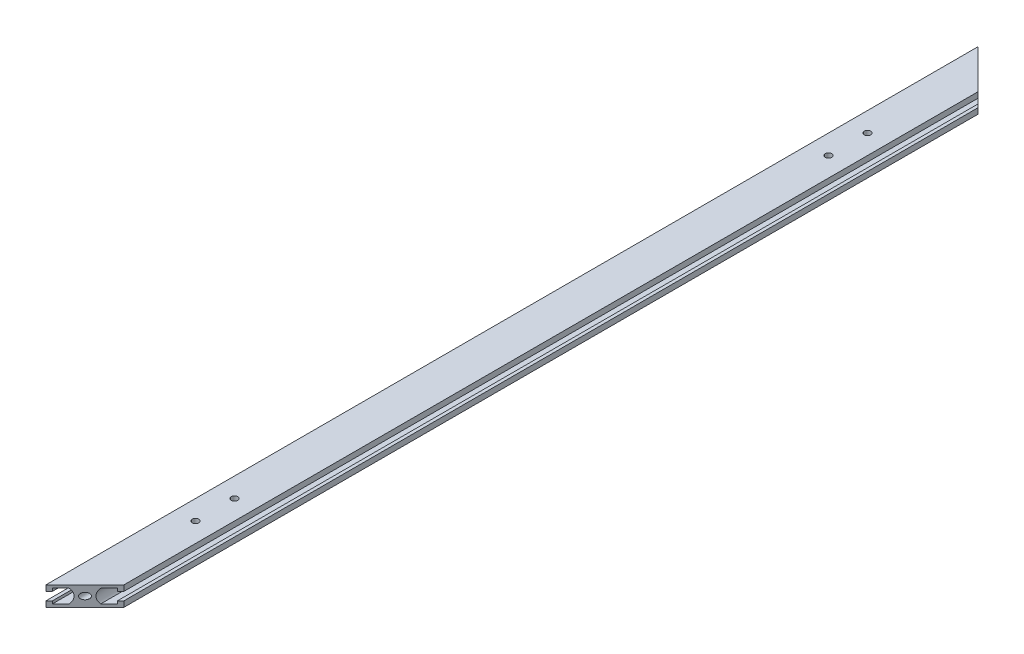
SolidWorks part; units mm, degrees
material "铝型材"
ref_plane "前视基准面" through (0, 0, 0) normal (0, 0, 1) x (1, 0, 0)
ref_plane "上视基准面" through (0, 0, 0) normal (0, 1, 0) x (1, 0, 0)
ref_plane "右视基准面" through (0, 0, 0) normal (1, 0, 0) x (0, 0, -1)
sketch "Model" plane through (0, 0, 0) normal (0, 0, 1) x (1, 0, 0)
  line L0 (2390.4271, 419.7568) -> (2392.9271, 419.7568)
  line L1 (2390.4271, 419.7568) -> (2390.4271, 417.7068)
  line L2 (2392.9271, 415.4068) -> (2392.9271, 419.7568)
  line L3 (2383.9948, 417.7068) -> (2390.4271, 417.7068)
  line L4 (2362.9271, 415.4068) -> (2392.9271, 415.4068)
  line L5 (2362.9271, 415.4068) -> (2362.9271, 419.7568)
  line L6 (2383.9948, 428.1068) -> (2390.4271, 428.1068)
  line L7 (2365.4271, 419.7568) -> (2362.9271, 419.7568)
  line L8 (2390.4271, 426.0568) -> (2390.4271, 428.1068)
  line L9 (2365.4271, 419.7568) -> (2365.4271, 417.7068)
  line L10 (2390.4271, 426.0568) -> (2392.9271, 426.0568)
  line L11 (2365.4271, 417.7068) -> (2371.8571, 417.7068)
  line L12 (2392.9271, 430.4068) -> (2392.9271, 426.0568)
  line L13 (2362.9271, 430.4068) -> (2392.9271, 430.4068)
  line L14 (2365.4271, 428.1068) -> (2371.8571, 428.1068)
  line L15 (2362.9271, 430.4068) -> (2362.9271, 426.0568)
  line L16 (2365.4271, 426.0568) -> (2365.4271, 428.1068)
  line L17 (2365.4271, 426.0568) -> (2362.9271, 426.0568)
  line L22 (2361.3714, 422.9068) -> (2394.2123, 422.9068) construction
  line L23 (2377.9271, 430.4068) -> (2377.9271, 415.4068) construction
  arc A0 (2371.8571, 428.1068) -> (2371.8571, 417.7068) centre (2365.5621, 422.9068) cw
  arc A1 (2383.9948, 428.1068) -> (2383.9948, 417.7068) centre (2390.2996, 422.9068) ccw
  circle A4 centre (2377.9271, 422.9068) radius 2.5
  point P2 (2373.7271, 422.9068)
  point P3 (2382.1271, 422.9068)
  dimension "D3" = 4.2
  dimension "D8" = 5
  dimension "D12" = 4.2
  dimension "D1" = 30
  dimension "D2" = 2.5
  dimension "D4" = 6.43
  dimension "D5" = 6.3
  dimension "D6" = 10.4
  dimension "D7" = 15
  dimension "D9" = 6.3
  dimension "D10" = 2.5
  dimension "D11" = 6.4323
extrude "凸台-拉伸1" add sketch "Model" along normal mid plane 717 contours L13 L12 L10 L8 L6 A1 L3 L1 L0 L2 L4 L5 L7 L9 L11 A0 L14 L16 L17 L15 | A4
ref_plane "基准面1" through (2382.1271, 0, 0) normal (1, 0, 0) x (0, 0, -1)
ref_plane "基准面2" through (2373.7271, 0, 0) normal (-1, 0, 0) x (0, 0, 1)
ref_plane "基准面3" through (0, 422.9068, 0) normal (0, 1, 0) x (1, 0, 0)
ref_plane "基准面4" through (2377.9271, 0, 0) normal (-1, 0, 0) x (0, 0, 1)
sketch "草图1" plane through (0, 430.4068, 0) normal (0, 1, 0) x (1, 0, 0)
  line L0 (2362.9271, 358.5) -> (2392.9271, 328.5)
  line L1 (2392.9271, -358.5) -> (2392.9271, 358.5) construction
  line L2 (2392.9271, 328.5) -> (2392.9271, 358.5)
  line L3 (2392.9271, 358.5) -> (2362.9271, 358.5)
  line L4 (2362.9271, -358.5) -> (2392.9271, -328.5)
  line L5 (2392.9271, -328.5) -> (2392.9271, -358.5)
  line L6 (2392.9271, -358.5) -> (2362.9271, -358.5)
extrude "切除-拉伸1" cut sketch "草图1" against normal through all
hole_wizard "M6 螺纹孔1" positions "草图3" profile "草图2" tap size "M6" standard "GB" end condition through all
sketch "草图3" plane through (0, 430.4068, 0) normal (0, 1, 0) x (1, 0, 0)
  line L0 (2362.9271, -358.5) -> (2362.9271, 358.5) construction
  line L1 (2377.9271, 258.5) -> (2377.9271, 228.5) construction
  line L2 (2377.9271, 228.5) -> (2377.9271, -228.5) construction
  line L5 (2362.9271, 0) -> (2377.9271, 0) construction
  line L8 (2377.9271, -258.5) -> (2377.9271, -228.5) construction
  point P0 (2377.9271, -258.5)
  point P2 (2377.9271, -228.5)
  point P4 (2377.9271, 228.5)
  point P6 (2377.9271, 258.5)
  dimension "D1" = 100
  dimension "D2" = 30
  dimension "D3" = 15
cosmetic thread "孔螺蚊线13" parameters "D2"=6
cosmetic thread "孔螺蚊线14" parameters "D2"=6
cosmetic thread "孔螺蚊线15" parameters "D2"=6
cosmetic thread "孔螺蚊线16" parameters "D2"=6
sketch "草图2" plane through (2377.9271, 430.4068, 258.5) normal (1, 0, 0) x (0, 0, 1)
  line L0 (0, 0) -> (0, 15)
  line L1 (0, 15) -> (2.5, 15)
  line L2 (2.5, 15) -> (2.5, 0)
  line L5 (2.5, 0) -> (0, 0)
  line L11 (0, -6.35) -> (0, 107.95) construction
  dimension "通孔螺纹孔钻头直径" = 5
  dimension "通孔螺纹孔钻头深度" = 15
